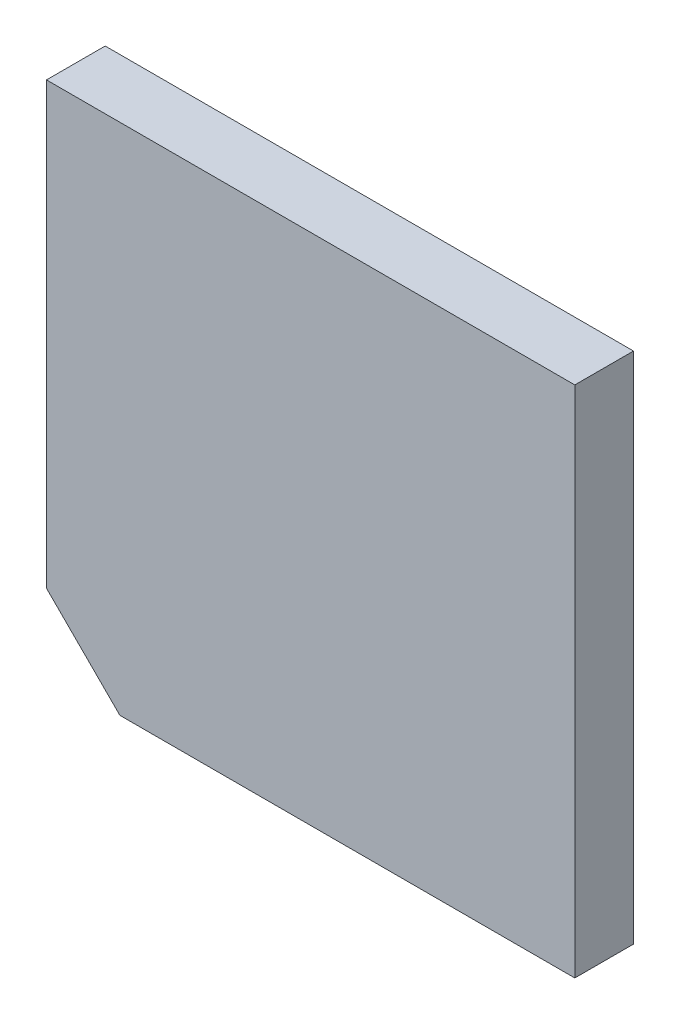
SolidWorks part; units mm, degrees
material "Q235A"
ref_plane "Front Plane" through (0, 0, 0) normal (0, 0, 1) x (1, 0, 0)
ref_plane "Top Plane" through (0, 0, 0) normal (0, 1, 0) x (1, 0, 0)
ref_plane "Right Plane" through (0, 0, 0) normal (1, 0, 0) x (0, 0, -1)
sketch "Sketch1" plane through (0, 0, 0) normal (0, 0, 1) x (1, 0, 0)
  line L0 (0, 0) -> (0, 35)
  line L1 (0, 35) -> (36, 35)
  line L2 (36, 35) -> (36, 0)
  line L3 (36, 0) -> (0, 0)
  dimension "D1" = 35
  dimension "D2" = 90
  dimension "D3" = 36
extrude "Boss-Extrude1" add sketch "Sketch1" along normal blind 4
chamfer "Chamfer1" distance 5 angle 45 1 edges at (0, 0, 2)
